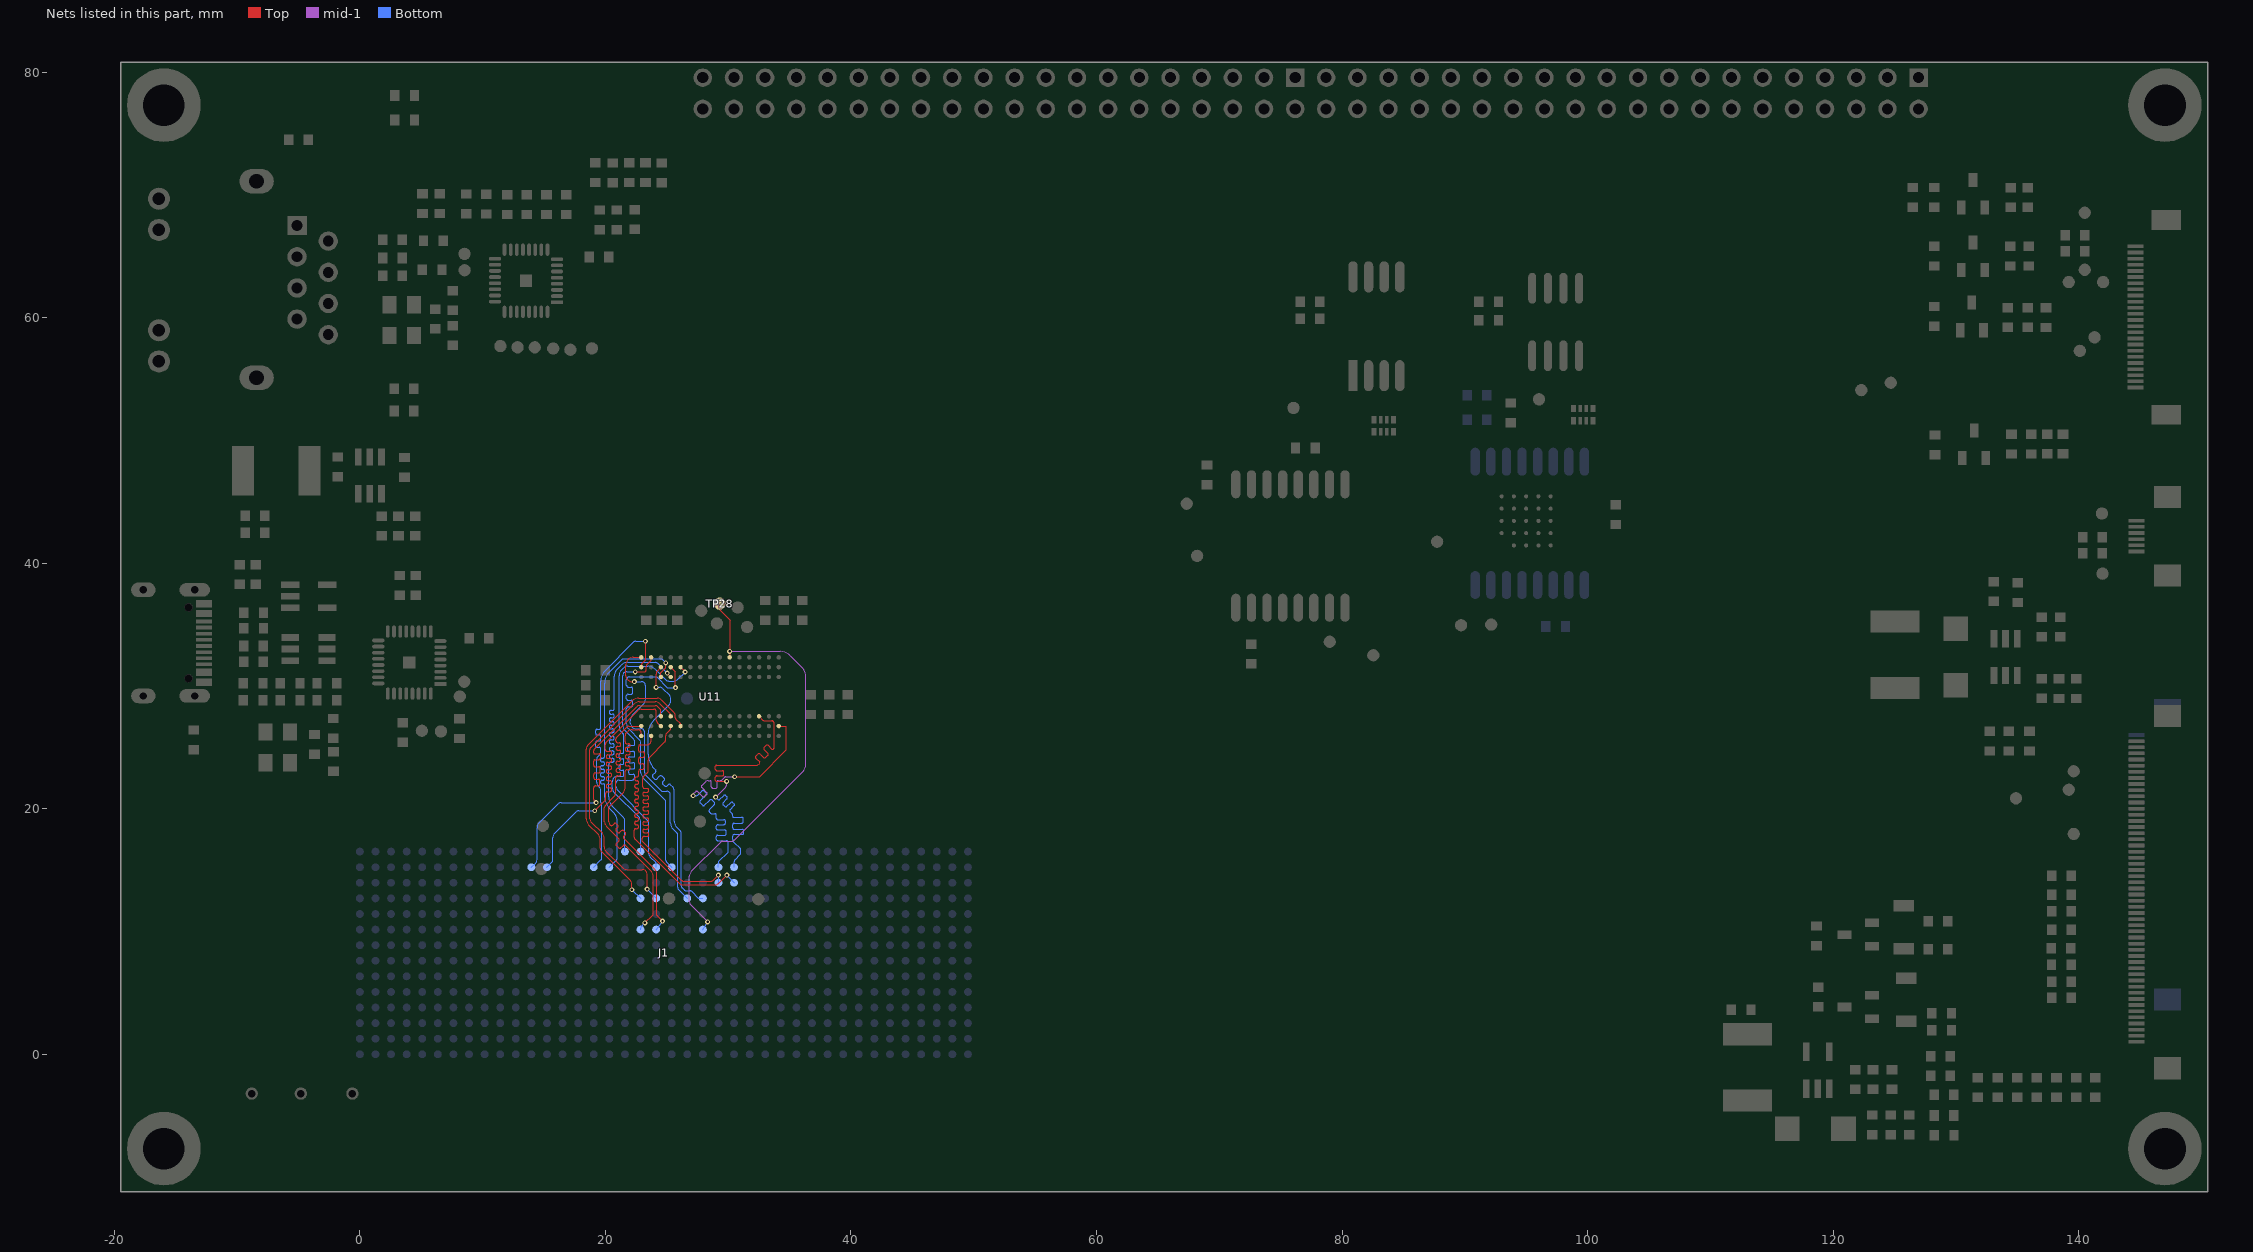
[diagram p0: the nets of this part, all layers, seen from the top]
# Altium PCB MISC105414.PcbDoc (part 10 of 11)
Units mm, origin at the board's own origin, x right, y up, seen from the top; angles counter-clockwise.
Board outline 170 x 92 mm, 6 copper layers (Top, GND, mid-1, mid-2, mid-3, Bottom), stack 1.231 mm thick; 238 components, 304 nets, 1456 pads, 1258 vias.
Unrouted connection lines stored in the file: 57.

## Via types
v1: diameter 0.4, hole 0.2, Top to Bottom, tented top, 618 vias
v2: diameter 0.5, hole 0.3, Top to Bottom, tented top, 522 vias
v3: diameter 0.5, hole 0.3, Top to Bottom, 41 vias
v4: diameter 1, hole 0.5, Top to Bottom, tented top, 36 vias
v5: diameter 0.7, hole 0.4, Top to Bottom, tented top, 34 vias
v6: diameter 1.3, hole 1.3, Top to Bottom, tented top, 3 vias
v7: diameter 4, hole 4, Top to Bottom, tented top, 2 vias
v8: diameter 3.3, hole 3.3, Top to Bottom, tented top, 2 vias

## Nets (pads, with @x,y where several pads share a name; then routed paths per layer and width w, separated by ;. In a path a pad name is that pad's centre, name@x,y a point inside that pad or via, vN(x,y) a via of type N, cw(c..) or ccw(c..) an arc to the next point about the centre after c; other vN are vias at no path point) (continued)
SDR_D14: J1.L16 U11.N3 | length 28.2
  Top w0.1: v1(29.874,22.224) 29.069,22.224 cw(c29.069,22.331) 28.962,22.331 28.962,22.558 cw(c29.098,22.558) 29.098,22.694 29.55,22.694 ccw(c29.55,22.788) 29.645,22.788 29.645,22.972 ccw(c29.516,22.972) 29.516,23.1 29.082,23.1 cw(c29.082,23.22) 28.962,23.22 28.962,23.454 cw(c29.054,23.454) 29.054,23.546 32.278,23.546 ccw(c32.278,23.875) 32.511,23.642 ; 32.511,23.642 32.556,23.688 ccw(c32.49,23.754) 32.584,23.754 ccw(c32.49,23.754) 32.556,23.82 32.25,24.126 cw(c32.333,24.21) 32.215,24.21 cw(c32.333,24.21) 32.25,24.293 32.417,24.46 cw(c32.504,24.372) 32.592,24.46 32.853,24.199 ccw(c32.96,24.306) 33.068,24.199 33.234,24.366 ccw(c33.163,24.437) 33.264,24.437 ccw(c33.163,24.437) 33.234,24.509 32.923,24.82 cw(c33.01,24.906) 32.887,24.906 cw(c33.01,24.906) 32.923,24.993 33.084,25.153 cw(c33.166,25.072) 33.247,25.153 33.527,24.874 ccw(c33.615,24.962) 33.739,24.962 33.739,26.975 ccw(c33.556,26.975) 33.556,27.158 32.982,27.158 cw(c32.982,27.369) 32.833,27.22 U11.N3@32.52,27.533
  mid-1 w0.1: v1(28.972,20.942) 29.79,21.76 ccw(c29.587,21.963) 29.874,21.963 v1(29.874,22.224)
  Bottom w0.1: v1(28.972,20.942) 29.157,20.757 ccw(c29.234,20.834) 29.311,20.757 29.622,21.067 cw(c29.714,20.976) 29.805,21.068 29.901,20.972 cw(c29.814,20.886) 29.937,20.886 cw(c29.814,20.886) 29.901,20.799 29.583,20.481 ccw(c29.658,20.406) 29.552,20.406 ccw(c29.658,20.406) 29.583,20.331 29.728,20.186 ccw(c29.814,20.272) 29.899,20.186 30.218,20.505 cw(c30.303,20.42) 30.387,20.505 30.501,20.391 cw(c30.448,20.338) 30.523,20.338 cw(c30.448,20.338) 30.501,20.285 30.151,19.935 ccw(c30.237,19.849) 30.116,19.849 ccw(c30.237,19.849) 30.151,19.763 30.149,19.761 30.311,19.598 cw(c30.195,19.482) 30.36,19.482 30.36,19.382 ccw(c30.442,19.382) 30.442,19.3 31.109,19.3 cw(c31.109,19.175) 31.234,19.175 31.234,18.967 cw(c31.098,18.967) 31.098,18.831 30.506,18.831 ccw(c30.506,18.685) 30.36,18.685 30.36,18.459 ccw(c30.501,18.459) 30.501,18.318 31.168,18.318 cw(c31.168,18.221) 31.265,18.221 31.265,18.017 cw(c31.155,18.017) 31.155,17.907 30.504,17.907 ccw(c30.504,17.763) 30.36,17.763 30.36,17.522 ccw(c30.722,17.522) 30.466,17.266 30.966,16.765 cw(c30.792,16.592) 31.038,16.592 31.038,16.42 cw(c30.832,16.42) 30.978,16.275 30.559,15.857 ccw(c30.75,15.666) 30.48,15.666 J1.L16@30.48,15.24
SDR_D15: J1.L17 U11.R2 | length 27.9
  Top w0.1: v1(30.517,22.609) 30.517,22.608 32.559,22.608 34.749,24.798 34.749,26.733 U11.R2@34.12,26.733
  mid-1 w0.1: v1(27.139,21.056) 27.139,21.097 cw(c27.357,21.097) 27.203,21.251 27.34,21.389 cw(c27.422,21.307) 27.503,21.389 27.886,21.006 ccw(c27.993,21.113) 28.1,21.006 28.273,21.179 ccw(c28.208,21.244) 28.3,21.244 ccw(c28.208,21.244) 28.273,21.309 27.843,21.74 cw(c27.918,21.815) 27.811,21.815 cw(c27.918,21.815) 27.842,21.891 28.156,22.205 cw(c28.371,21.989) 28.371,22.294 28.52,22.294 cw(c28.52,22.182) 28.632,22.182 28.632,21.776 ccw(c28.724,21.776) 28.724,21.684 29.025,21.684 ccw(c29.025,21.755) 29.096,21.755 29.096,22.206 cw(c29.184,22.206) 29.184,22.294 29.336,22.294 ccw(c29.336,22.522) 29.497,22.361 29.704,22.567 cw(c29.805,22.466) 29.805,22.609 v1(30.517,22.609)
  Bottom w0.1: v1(27.139,21.056) 27.375,21.056 ccw(c27.375,21.237) 27.503,21.109 27.839,21.445 cw(c27.949,21.335) 28.059,21.445 28.21,21.294 cw(c28.129,21.213) 28.243,21.213 cw(c28.129,21.213) 28.21,21.133 27.716,20.639 ccw(c27.796,20.559) 27.683,20.559 ccw(c27.796,20.559) 27.716,20.479 27.91,20.285 ccw(c27.99,20.364) 28.069,20.285 28.48,20.696 cw(c28.592,20.583) 28.705,20.696 28.868,20.533 cw(c28.769,20.434) 28.909,20.434 cw(c28.769,20.434) 28.868,20.335 28.479,19.946 ccw(c28.594,19.831) 28.431,19.831 ccw(c28.594,19.831) 28.479,19.716 28.531,19.664 ccw(c28.697,19.829) 28.697,19.595 28.908,19.595 cw(c28.908,19.466) 29.038,19.466 29.038,19.213 ccw(c29.138,19.213) 29.138,19.113 29.644,19.113 cw(c29.644,18.976) 29.781,18.976 29.781,18.853 cw(c29.643,18.853) 29.643,18.714 29.185,18.714 ccw(c29.185,18.567) 29.038,18.567 29.038,18.385 ccw(c29.148,18.385) 29.148,18.275 29.707,18.275 cw(c29.707,18.14) 29.842,18.14 29.842,17.963 cw(c29.734,17.963) 29.734,17.855 29.156,17.855 ccw(c29.156,17.736) 29.038,17.736 29.038,17.505 ccw(c29.13,17.505) 29.13,17.413 29.856,17.413 cw(c29.856,17.276) 29.993,17.276 29.993,16.457 29.246,15.71 J1.L17@29.21,15.24
SDR_D16: J1.M22 U11.E8 | length 24.4
  Top w0.1: U11.E8@26.12,31.533 26.488,31.165 v1(26.488,31.139)
  Bottom w0.1: J1.M22@22.86,16.51 22.86,19.028 ccw(c22.461,19.028) 22.743,19.31 20.695,21.358 cw(c21.029,21.693) 20.557,21.693 20.557,22.196 cw(c20.995,22.196) 20.995,22.634 21.393,22.634 ccw(c21.393,22.751) 21.509,22.751 21.509,23.054 ccw(c21.407,23.054) 21.407,23.157 21.238,23.157 cw(c21.238,23.278) 21.117,23.278 21.117,23.494 cw(c21.24,23.494) 21.24,23.617 21.399,23.617 ccw(c21.399,23.727) 21.509,23.727 21.509,23.962 ccw(c21.4,23.962) 21.4,24.072 21.214,24.072 cw(c21.214,24.164) 21.121,24.164 21.121,24.435 cw(c21.215,24.435) 21.215,24.529 21.401,24.529 ccw(c21.401,24.637) 21.509,24.637 21.509,25.913 ccw(c21.206,25.913) 21.42,26.128 21.315,26.233 cw(c21.811,26.728) 21.11,26.728 21.11,30.85 cw(c21.703,30.85) 21.284,31.269 21.5,31.486 cw(c21.814,31.172) 21.814,31.616 23.462,31.616 cw(c23.462,30.798) 24.04,31.376 24.902,30.514 ccw(c25.164,30.775) 25.164,30.405 25.569,30.405 ccw(c25.569,30.851) 25.884,30.536 v1(26.488,31.139)
SDR_D17: J1.M23 U11.D7 | length 24.8
  Top w0.1: v1(25.038,31.052) 25.038,31.014 U11.D7@25.32,30.733
  Bottom w0.1: J1.M23@21.59,16.51 21.59,18.994 ccw(c21.155,18.994) 21.463,19.302 20.574,20.19 cw(c21.346,20.962) 20.255,20.962 20.255,23.592 cw(c20.469,23.592) 20.469,23.806 20.57,23.806 ccw(c20.57,23.956) 20.72,23.956 ccw(c20.57,23.956) 20.57,24.106 20.457,24.106 cw(c20.457,24.256) 20.307,24.256 cw(c20.457,24.256) 20.457,24.406 20.57,24.406 ccw(c20.57,24.556) 20.72,24.556 ccw(c20.57,24.556) 20.57,24.706 20.457,24.706 cw(c20.457,24.856) 20.307,24.856 cw(c20.457,24.856) 20.457,25.006 20.57,25.006 ccw(c20.57,25.156) 20.72,25.156 ccw(c20.57,25.156) 20.57,25.306 20.457,25.306 cw(c20.457,25.456) 20.307,25.456 cw(c20.457,25.456) 20.457,25.606 20.57,25.606 ccw(c20.57,25.756) 20.72,25.756 ccw(c20.57,25.756) 20.57,25.906 20.457,25.906 cw(c20.457,26.056) 20.307,26.056 cw(c20.457,26.056) 20.457,26.206 20.57,26.206 ccw(c20.57,26.356) 20.72,26.356 ccw(c20.57,26.356) 20.57,26.506 20.457,26.506 cw(c20.457,26.656) 20.307,26.656 cw(c20.457,26.656) 20.457,26.806 20.57,26.806 ccw(c20.57,26.956) 20.72,26.956 ccw(c20.57,26.956) 20.57,27.106 20.457,27.106 cw(c20.457,27.256) 20.307,27.256 cw(c20.457,27.256) 20.457,27.406 20.57,27.406 ccw(c20.57,27.556) 20.72,27.556 ccw(c20.57,27.556) 20.57,27.706 20.457,27.706 cw(c20.457,27.856) 20.307,27.856 cw(c20.457,27.856) 20.457,28.006 20.57,28.006 ccw(c20.57,28.156) 20.72,28.156 20.72,30.784 cw(c21.56,30.784) 20.966,31.378 21.289,31.701 cw(c21.809,31.182) 21.809,31.916 24.063,31.916 cw(c24.063,31.648) 24.253,31.838 v1(25.038,31.052)
SDR_D18: J1.L20 U11.D8 | length 24.6
  Top w0.1: U11.D8@25.32,31.533 25.7,31.153 25.7,29.867 v1(25.71,29.867)
  Bottom w0.1: J1.L20@25.4,15.24 24.992,15.648 cw(c25.141,15.798) 24.93,15.798 24.93,20.532 ccw(c24.653,20.532) 24.849,20.727 23.05,22.526 cw(c23.451,22.927) 22.884,22.927 22.884,25.347 ccw(c22.481,25.347) 22.766,25.632 21.894,26.505 cw(c22.322,26.932) 21.717,26.932 21.717,28.159 cw(c21.872,28.159) 21.872,28.314 22.121,28.314 ccw(c22.121,28.401) 22.209,28.401 22.209,28.723 ccw(c22.093,28.723) 22.093,28.839 21.825,28.839 cw(c21.825,28.947) 21.717,28.947 21.717,29.204 cw(c21.853,29.204) 21.853,29.341 22.119,29.341 ccw(c22.119,29.441) 22.219,29.441 22.219,29.783 ccw(c22.095,29.783) 22.095,29.908 21.883,29.908 cw(c21.883,30.073) 21.717,30.073 21.717,30.503 cw(c21.96,30.503) 21.96,30.746 24.164,30.746 25.043,29.867 v1(25.71,29.867)
SDR_D19: J1.L21 U11.B9 | length 24.6
  Top w0.1: v1(22.428,31.151) 23.183,31.151 ccw(c23.183,31.287) 23.32,31.287 23.32,31.599 cw(c23.514,31.599) 23.377,31.737 23.689,32.049 ; 23.689,32.049 ccw(c23.614,32.124) 23.72,32.124 U11.B9@23.72,32.333
  Bottom w0.1: v1(22.428,31.151) 21.723,31.151 ccw(c21.723,30.838) 21.41,30.838 21.41,26.776 ccw(c21.926,26.776) 21.561,26.412 22.253,25.72 cw(c21.914,25.381) 22.394,25.381 22.394,25.255 cw(c22.306,25.255) 22.306,25.167 21.947,25.167 ccw(c21.947,25.03) 21.81,25.03 21.81,24.77 ccw(c21.912,24.77) 21.912,24.668 22.237,24.668 cw(c22.237,24.511) 22.394,24.511 22.394,24.303 cw(c22.308,24.303) 22.308,24.217 21.94,24.217 ccw(c21.94,24.124) 21.846,24.124 21.846,23.862 ccw(c21.942,23.862) 21.942,23.766 22.243,23.766 cw(c22.243,23.615) 22.394,23.615 22.394,23.378 cw(c22.257,23.378) 22.257,23.241 22.032,23.241 ccw(c22.032,23.091) 21.882,23.091 21.882,22.916 ccw(c21.999,22.916) 21.999,22.8 22.267,22.8 cw(c22.267,22.673) 22.394,22.673 22.394,22.579 cw(c22.148,22.579) 22.148,22.333 21.125,22.333 ccw(c21.125,22.066) 20.857,22.066 20.857,21.835 ccw(c21.303,21.835) 20.988,21.52 23.468,19.04 cw(c23.312,18.884) 23.532,18.884 23.532,16.348 ccw(c23.868,16.348) 23.63,16.11 24.094,15.647 cw(c24.006,15.559) 24.13,15.559 J1.L21@24.13,15.24
SDR_D20: J1.J18 U11.C8 | length 24.1
  Top w0.1: v1(24.128,29.888) 24.129,29.849 24.129,30.976 cw(c24.529,30.976) 24.246,31.259 U11.C8@24.52,31.533
  Bottom w0.1: v1(24.128,29.888) 24.443,29.888 cw(c24.443,29.55) 24.681,29.789 25.199,29.271 cw(c24.912,28.985) 25.317,28.985 25.317,28.735 cw(c24.971,28.735) 25.216,28.49 23.926,27.2 ccw(c24.972,26.154) 23.492,26.154 23.492,24.448 ccw(c25.15,24.448) 23.978,23.276 24.079,23.174 cw(c23.977,23.072) 24.122,23.072 cw(c23.977,23.072) 24.079,22.969 23.867,22.756 ccw(c23.966,22.657) 23.825,22.657 ccw(c23.966,22.657) 23.867,22.558 24.003,22.422 ccw(c24.094,22.514) 24.186,22.422 24.397,22.633 cw(c24.509,22.521) 24.621,22.633 ; 24.621,22.633 24.788,22.465 cw(c24.709,22.386) 24.821,22.386 cw(c24.709,22.386) 24.788,22.306 24.68,22.198 ccw(c24.782,22.096) 24.638,22.096 ccw(c24.782,22.096) 24.68,21.994 24.815,21.859 ccw(c24.921,21.966) 25.028,21.859 25.121,21.953 cw(c25.211,21.863) 25.301,21.953 25.478,21.776 ; 25.478,21.776 cw(c25.181,21.478) 25.601,21.478 25.601,18.985 ccw(c26.302,18.985) 25.807,18.489 26.099,18.196 cw(c25.907,18.004) 26.179,18.004 26.179,13.712 ccw(c26.406,13.712) 26.246,13.551 26.403,13.394 ccw(c26.582,13.572) 26.582,13.32 26.879,13.32 cw(c26.879,13.128) 27.015,13.263 27.528,12.75 ccw(c27.648,12.87) 27.648,12.7 J1.J18@27.94,12.7
SDR_D21: J1.J19 U11.A9 | length 24.8
  Top w0.1: v1(22.364,30.357) 22.146,30.357 cw(c22.146,30.843) 21.661,30.843 21.661,31.724 cw(c22.27,31.724) 22.27,32.333 U11.A9@22.92,32.333
  Bottom w0.1: v1(22.364,30.357) 22.931,30.357 cw(c22.931,30.021) 23.267,30.021 23.267,28.939 cw(c22.686,28.939) 23.097,28.529 22.237,27.669 ccw(c22.73,27.176) 22.033,27.176 22.033,26.985 ccw(c22.499,26.985) 22.499,26.518 22.893,26.518 cw(c22.893,26.222) 23.189,26.222 23.189,22.924 ccw(c23.461,22.924) 23.269,22.731 24.57,21.431 24.993,21.431 cw(c24.993,21.13) 25.294,21.13 25.294,18.841 ccw(c25.934,18.841) 25.481,18.389 25.827,18.043 cw(c25.703,17.918) 25.879,17.918 25.879,13.61 ccw(c26.164,13.61) 25.962,13.408 J1.J19@26.67,12.7
SDR_D22: J1.L24 U11.C7 | length 24.9
  Top w0.1: U11.C7@24.52,30.733 24.52,31.069 24.926,31.475 24.926,31.872 v1(24.916,31.881)
  Bottom w0.1: J1.L24@20.32,15.24 20.87,15.79 ccw(c20.613,16.047) 20.977,16.047 20.977,19.004 ccw(c20.109,19.004) 20.723,19.617 20.345,19.995 cw(c21.289,20.939) 19.954,20.939 19.954,21.925 ccw(c19.858,21.925) 19.858,22.02 19.733,22.02 cw(c19.733,22.17) 19.583,22.17 cw(c19.733,22.17) 19.733,22.32 19.788,22.32 ccw(c19.788,22.47) 19.938,22.47 ccw(c19.788,22.47) 19.788,22.62 19.733,22.62 cw(c19.733,22.77) 19.583,22.77 cw(c19.733,22.77) 19.733,22.92 19.788,22.92 ccw(c19.788,23.07) 19.938,23.07 ccw(c19.788,23.07) 19.788,23.22 19.733,23.22 cw(c19.733,23.37) 19.583,23.37 cw(c19.733,23.37) 19.733,23.52 19.788,23.52 ccw(c19.788,23.67) 19.938,23.67 ccw(c19.788,23.67) 19.788,23.82 19.733,23.82 cw(c19.733,23.97) 19.583,23.97 cw(c19.733,23.97) 19.733,24.12 19.788,24.12 ccw(c19.788,24.27) 19.938,24.27 19.938,30.241 cw(c21.139,30.241) 20.29,31.091 21.419,32.219 24.578,32.219 v1(24.916,31.881)
SDR_D23: J1.L25 U11.A8 | length 24.5
  Top w0.1: U11.A8@22.92,31.533 22.92,31.709 cw(c23.059,31.709) 22.961,31.807 23.234,32.08 ccw(c23.094,32.221) 23.292,32.221 23.292,33.484 23.3,33.491 23.279,33.512 23.269,33.565 v1(23.253,33.648)
  Bottom w0.1: J1.L25@19.05,15.24 19.64,15.83 ccw(c19.449,16.021) 19.719,16.021 19.719,20.309 ccw(c19.57,20.309) 19.675,20.414 19.667,20.421 cw(c19.772,20.526) 19.624,20.526 19.624,21.49 ccw(c19.255,21.49) 19.516,21.751 19.397,21.87 cw(c19.688,22.161) 19.276,22.161 19.276,24.037 cw(c19.574,24.037) 19.363,24.247 19.525,24.409 ccw(c19.311,24.622) 19.613,24.622 19.613,24.9 ccw(c19.511,24.9) 19.511,25.002 19.274,25.002 cw(c19.274,25.081) 19.195,25.081 19.195,25.386 cw(c19.328,25.386) 19.328,25.52 19.509,25.52 ccw(c19.509,25.648) 19.638,25.648 19.638,25.91 ccw(c19.537,25.91) 19.537,26.011 19.319,26.011 cw(c19.319,26.134) 19.196,26.134 19.196,26.358 cw(c19.323,26.358) 19.323,26.485 19.516,26.485 ccw(c19.516,26.583) 19.613,26.583 19.613,30.391 cw(c20.78,30.391) 19.955,31.216 22.328,33.589 cw(c22.469,33.447) 22.469,33.648 v1(23.253,33.648)
SDR_D24: J1.G22 U11.A2 | length 24.1
  Top w0.1: U11.A2@22.92,26.733 21.916,26.733 ccw(c21.916,26.523) 21.768,26.671 20.905,25.809 ccw(c21.043,25.671) 20.848,25.671 20.848,25.539 20.855,25.531 ccw(c21.005,25.531) 21.005,25.381 21.115,25.381 cw(c21.115,25.231) 21.265,25.231 cw(c21.115,25.231) 21.115,25.081 21.005,25.081 ccw(c21.005,24.931) 20.855,24.931 ccw(c21.005,24.931) 21.005,24.781 21.115,24.781 cw(c21.115,24.631) 21.265,24.631 cw(c21.115,24.631) 21.115,24.481 21.005,24.481 ccw(c21.005,24.331) 20.855,24.331 ccw(c21.005,24.331) 21.005,24.181 21.115,24.181 cw(c21.115,24.031) 21.265,24.031 cw(c21.115,24.031) 21.115,23.881 21.005,23.881 ccw(c21.005,23.731) 20.855,23.731 ccw(c21.005,23.731) 21.005,23.581 21.115,23.581 cw(c21.115,23.431) 21.265,23.431 cw(c21.115,23.431) 21.115,23.281 21.005,23.281 ccw(c21.005,23.131) 20.855,23.131 ccw(c21.005,23.131) 21.005,22.981 21.115,22.981 cw(c21.115,22.831) 21.265,22.831 cw(c21.115,22.831) 21.115,22.681 20.999,22.681 ccw(c20.999,22.531) 20.849,22.531 20.849,21.365 cw(c20.274,21.365) 20.681,20.959 20.012,20.291 ccw(c20.232,20.071) 19.921,20.071 19.921,18.951 ccw(c20.436,18.951) 20.072,18.587 21.089,17.57 cw(c20.982,17.464) 21.133,17.464 cw(c20.982,17.464) 21.089,17.357 20.871,17.139 ccw(c20.935,17.074) 20.844,17.074 ccw(c20.935,17.074) 20.871,17.01 21.069,16.812 ccw(c21.16,16.903) 21.251,16.812 21.436,16.997 cw(c21.549,16.884) 21.662,16.997 23.701,14.958 cw(c23.22,14.478) 23.9,14.478 23.9,11.465 cw(c23.688,11.465) 23.838,11.315 v1(23.221,10.698)
  Bottom w0.1: J1.G22@22.86,10.16 22.86,10.268 cw(c23.026,10.268) 22.909,10.385 v1(23.221,10.698)
SDR_D25: J1.L29 U11.C3 | length 23.8
  Top w0.1: v1(19.242,20.501) 19.072,20.671 cw(c19.175,20.774) 19.029,20.774 19.029,21.692 cw(c19.193,21.692) 19.193,21.856 19.413,21.856 ccw(c19.413,21.989) 19.545,21.989 19.545,22.293 ccw(c19.431,22.293) 19.431,22.408 19.169,22.408 cw(c19.169,22.547) 19.029,22.547 19.029,22.779 cw(c19.172,22.779) 19.172,22.922 19.475,22.922 ccw(c19.475,23.02) 19.572,23.02 19.572,23.332 ccw(c19.471,23.332) 19.471,23.433 19.133,23.433 cw(c19.133,23.537) 19.029,23.537 19.029,23.877 cw(c19.148,23.877) 19.148,23.995 19.44,23.995 ccw(c19.44,24.155) 19.6,24.155 19.6,24.387 ccw(c19.495,24.387) 19.495,24.493 19.096,24.493 cw(c19.096,24.559) 19.029,24.559 19.029,24.712 cw(c19.2,24.712) 19.079,24.833 22.564,28.318 cw(c22.782,28.1) 22.782,28.408 24.079,28.408 cw(c24.079,28.192) 24.232,28.345 24.436,28.141 cw(c24.232,27.937) 24.52,27.937 U11.C3@24.52,27.533
  Bottom w0.1: J1.L29@13.97,15.24 14.308,15.578 ccw(c13.986,15.899) 14.441,15.899 14.441,18.47 cw(c14.986,18.47) 14.601,18.856 16.146,20.401 cw(c16.388,20.16) 16.388,20.501 v1(19.242,20.501)
SDR_D26: J1.G21 U11.A1 | length 23.8
  Top w0.1: 20.871,18.213 21.007,18.077 ccw(c21.091,18.162) 21.175,18.077 21.301,18.203 cw(c21.397,18.106) 21.493,18.203 21.634,18.062 cw(c21.546,17.973) 21.671,17.973 cw(c21.546,17.973) 21.634,17.885 21.503,17.754 ccw(c21.59,17.668) 21.467,17.668 ccw(c21.59,17.668) 21.503,17.581 24.01,15.074 cw(c23.551,14.615) 24.2,14.615 24.2,11.345 ccw(c24.309,11.345) 24.232,11.268 v1(24.65,10.85) ; 20.87,18.213 cw(c20.946,18.289) 20.839,18.289 cw(c20.946,18.289) 20.871,18.364 21.005,18.498 ccw(c20.925,18.578) 21.038,18.578 ccw(c20.925,18.578) 21.005,18.658 20.87,18.793 ccw(c20.791,18.714) 20.712,18.793 20.59,18.671 cw(c20.501,18.759) 20.413,18.67 20.367,18.717 cw(c20.577,18.928) 20.279,18.928 20.279,20.035 cw(c20.518,20.035) 20.349,20.203 21.406,21.26 ccw(c20.898,21.769) 21.617,21.769 21.617,23.042 cw(c21.767,23.042) 21.767,23.192 21.869,23.192 ccw(c21.869,23.342) 22.019,23.342 ccw(c21.869,23.342) 21.869,23.492 21.746,23.492 cw(c21.746,23.642) 21.596,23.642 cw(c21.746,23.642) 21.746,23.792 21.869,23.792 ccw(c21.869,23.942) 22.019,23.942 ccw(c21.869,23.942) 21.869,24.092 21.746,24.092 cw(c21.746,24.242) 21.596,24.242 cw(c21.746,24.242) 21.746,24.392 21.869,24.392 ccw(c21.869,24.542) 22.019,24.542 ccw(c21.869,24.542) 21.869,24.692 21.746,24.692 cw(c21.746,24.842) 21.596,24.842 cw(c21.746,24.842) 21.746,24.992 21.869,24.992 ccw(c21.869,25.142) 22.019,25.142 ccw(c21.869,25.142) 21.869,25.292 21.746,25.292 cw(c21.746,25.442) 21.596,25.442 21.596,25.964 cw(c21.861,25.964) 21.673,26.152 21.803,26.282 cw(c22.191,25.858) 22.191,26.433 22.674,26.433 cw(c22.674,26.186) 22.92,26.186 U11.A1@22.92,25.933
  Bottom w0.1: J1.G21@24.13,10.16 v1(24.65,10.85)
SDR_D27: J1.L28 U11.C2 | length 23.7
  Top w0.1: v1(19.133,19.836) 19.975,20.678 ccw(c19.869,20.785) 20.019,20.785 20.019,21.247 cw(c20.169,21.247) 20.169,21.397 20.363,21.397 ccw(c20.363,21.547) 20.513,21.547 ccw(c20.363,21.547) 20.363,21.697 20.198,21.697 cw(c20.198,21.847) 20.048,21.847 cw(c20.198,21.847) 20.198,21.997 20.363,21.997 ccw(c20.363,22.147) 20.513,22.147 ccw(c20.363,22.147) 20.363,22.297 20.198,22.297 cw(c20.198,22.447) 20.048,22.447 cw(c20.198,22.447) 20.198,22.597 20.363,22.597 ccw(c20.363,22.747) 20.513,22.747 ccw(c20.363,22.747) 20.363,22.897 20.198,22.897 cw(c20.198,23.047) 20.048,23.047 cw(c20.198,23.047) 20.198,23.197 20.363,23.197 ccw(c20.363,23.347) 20.513,23.347 ccw(c20.363,23.347) 20.363,23.497 20.198,23.497 cw(c20.198,23.647) 20.048,23.647 cw(c20.198,23.647) 20.198,23.797 20.363,23.797 ccw(c20.363,23.947) 20.513,23.947 ccw(c20.363,23.947) 20.363,24.097 20.198,24.097 cw(c20.198,24.247) 20.048,24.247 cw(c20.198,24.247) 20.198,24.397 20.363,24.397 ccw(c20.363,24.547) 20.513,24.547 ccw(c20.363,24.547) 20.363,24.697 20.122,24.697 cw(c20.122,24.847) 19.972,24.847 19.972,25.203 cw(c20.206,25.203) 20.04,25.368 22.694,28.022 cw(c22.899,27.816) 22.899,28.107 23.95,28.107 cw(c23.95,27.907) 24.15,27.907 24.15,27.221 ccw(c24.435,27.221) 24.233,27.019 U11.C2@24.52,26.733
  Bottom w0.1: J1.L28@15.24,15.24 15.714,15.714 15.714,17.654 cw(c16.169,17.654) 15.847,17.976 17.617,19.746 cw(c17.833,19.53) 17.833,19.836 v1(19.133,19.836)
SDR_D28: J1.K16 U11.B1 | length 24
  Top w0.1: 22.518,19.288 22.554,19.288 cw(c22.554,19.138) 22.704,19.138 cw(c22.554,19.138) 22.554,18.988 22.518,18.988 ccw(c22.518,18.838) 22.368,18.838 ccw(c22.518,18.838) 22.518,18.688 22.554,18.688 cw(c22.554,18.538) 22.704,18.538 cw(c22.554,18.538) 22.554,18.388 22.482,18.388 ccw(c22.482,18.238) 22.332,18.238 22.332,17.671 ccw(c22.495,17.671) 22.379,17.556 25.962,13.973 ccw(c26.389,14.399) 26.389,13.796 28.934,13.796 ccw(c28.934,14.188) 29.211,13.911 v1(29.9,14.6) ; 22.518,19.288 cw(c22.518,19.438) 22.368,19.438 cw(c22.518,19.438) 22.518,19.588 22.554,19.588 ccw(c22.554,19.738) 22.704,19.738 ccw(c22.554,19.738) 22.554,19.888 22.518,19.888 cw(c22.518,20.038) 22.368,20.038 cw(c22.518,20.038) 22.518,20.188 22.554,20.188 ccw(c22.554,20.338) 22.704,20.338 ccw(c22.554,20.338) 22.554,20.488 22.518,20.488 cw(c22.518,20.638) 22.368,20.638 cw(c22.518,20.638) 22.518,20.788 22.554,20.788 ccw(c22.554,20.938) 22.704,20.938 ccw(c22.554,20.938) 22.554,21.088 22.518,21.088 cw(c22.518,21.238) 22.368,21.238 cw(c22.518,21.238) 22.518,21.388 22.554,21.388 ccw(c22.554,21.538) 22.704,21.538 ccw(c22.554,21.538) 22.554,21.688 22.518,21.688 cw(c22.518,21.838) 22.368,21.838 cw(c22.518,21.838) 22.518,21.988 22.554,21.988 ccw(c22.554,22.138) 22.704,22.138 ccw(c22.554,22.138) 22.554,22.288 22.518,22.288 cw(c22.518,22.438) 22.368,22.438 cw(c22.518,22.438) 22.518,22.588 22.554,22.588 ccw(c22.554,22.738) 22.704,22.738 22.704,23.07 cw(c22.841,23.07) 22.841,23.207 22.992,23.207 ccw(c22.992,23.369) 23.154,23.369 23.154,23.533 ccw(c23.013,23.533) 23.013,23.675 22.805,23.675 cw(c22.805,23.775) 22.704,23.775 22.704,24.087 cw(c22.81,24.087) 22.81,24.193 23.067,24.193 ccw(c23.067,24.311) 23.185,24.311 23.185,24.521 ccw(c23.069,24.521) 23.069,24.636 22.784,24.636 cw(c22.784,24.716) 22.704,24.716 22.704,25.067 cw(c22.85,25.067) 22.85,25.213 23.389,25.213 ccw(c23.389,25.544) 23.72,25.544 U11.B1@23.72,25.933
  Bottom w0.1: v1(29.9,14.6) J1.K16@30.48,13.97
SDR_D29: J1.K17 U11.D2 | length 24.1
  Top w0.1: 23.183,21.65 23.399,21.65 cw(c23.399,21.5) 23.549,21.5 cw(c23.399,21.5) 23.399,21.35 23.183,21.35 ccw(c23.183,21.2) 23.033,21.2 ccw(c23.183,21.2) 23.183,21.05 23.399,21.05 cw(c23.399,20.9) 23.549,20.9 cw(c23.399,20.9) 23.399,20.75 23.183,20.75 ccw(c23.183,20.6) 23.033,20.6 ccw(c23.183,20.6) 23.183,20.45 23.399,20.45 cw(c23.399,20.3) 23.549,20.3 cw(c23.399,20.3) 23.399,20.15 23.183,20.15 ccw(c23.183,20) 23.033,20 ccw(c23.183,20) 23.183,19.85 23.399,19.85 cw(c23.399,19.7) 23.549,19.7 cw(c23.399,19.7) 23.399,19.55 23.183,19.55 ccw(c23.183,19.4) 23.033,19.4 ccw(c23.183,19.4) 23.183,19.25 23.399,19.25 cw(c23.399,19.1) 23.549,19.1 cw(c23.399,19.1) 23.399,18.95 23.183,18.95 ccw(c23.183,18.8) 23.033,18.8 ccw(c23.183,18.8) 23.183,18.65 23.399,18.65 cw(c23.399,18.5) 23.549,18.5 cw(c23.399,18.5) 23.399,18.35 23.183,18.35 ccw(c23.183,18.2) 23.033,18.2 ccw(c23.183,18.2) 23.183,18.05 23.399,18.05 cw(c23.399,17.9) 23.549,17.9 cw(c23.399,17.9) 23.399,17.75 23.157,17.75 ccw(c23.157,17.6) 23.007,17.6 23.007,17.353 26.165,14.194 ccw(c26.401,14.43) 26.401,14.097 28.616,14.097 ccw(c28.616,14.307) 28.765,14.159 v1(29.197,14.59) ; 23.183,21.65 cw(c23.183,21.8) 23.033,21.8 23.033,22.439 cw(c23.265,22.439) 23.101,22.603 23.417,22.92 ccw(c23.24,23.097) 23.491,23.097 23.491,23.943 cw(c23.86,23.943) 23.599,24.204 24.84,25.445 ccw(c24.694,25.591) 24.9,25.591 24.9,25.953 cw(c25.158,25.953) 24.976,26.135 25.281,26.44 ; 25.281,26.44 ccw(c25.186,26.535) 25.32,26.535 U11.D2@25.32,26.733
  Bottom w0.1: v1(29.197,14.59) J1.K17@29.21,13.97
SDR_D30: J1.J21 U11.D3 | length 23.9
  Top w0.1: v1(23.4,13.45) 23.4,14.653 ccw(c23.005,14.653) 23.005,15.048 21.785,15.048 cw(c21.785,15.632) 21.371,15.219 20.047,16.543 cw(c20.401,16.897) 19.901,16.897 19.901,17.606 ccw(c19.306,17.606) 19.726,18.027 18.848,18.905 cw(c19.137,19.193) 18.729,19.193 18.729,24.798 cw(c18.997,24.798) 18.808,24.987 22.36,28.539 cw(c22.769,28.13) 22.769,28.709 24.077,28.709 cw(c24.077,28.19) 24.444,28.557 25.32,27.681 U11.D3@25.32,27.533
  Bottom w0.1: v1(23.4,13.45) J1.J21@24.13,12.7
SDR_D31: J1.J22 U11.E2 | length 24.6
  Top w0.1: v1(22.15,13.4) 22.15,13.818 ccw(c21.67,13.818) 22.009,14.157 19.688,16.478 cw(c19.979,16.769) 19.568,16.769 19.568,17.487 ccw(c18.906,17.487) 19.374,17.955 18.621,18.708 cw(c19.085,19.172) 18.428,19.172 18.428,24.848 cw(c18.874,24.848) 18.559,25.163 22.189,28.793 cw(c22.711,28.271) 22.711,29.009 24.205,29.009 cw(c24.205,28.497) 24.568,28.859 25.569,27.858 cw(c25.264,27.552) 25.696,27.552 25.696,27.394 ccw(c25.815,27.394) 25.731,27.31 26.093,26.948 cw(c26.026,26.882) 26.12,26.882 U11.E2@26.12,26.733
  Bottom w0.1: v1(22.15,13.4) J1.J22@22.86,12.7
SDR_DQM0: J1.G18 TP28.1 U11.K9 | length 37.7
  Top w0.1: TP28.1@29.312,36.708 29.312,36.215 30.178,35.349 30.178,32.873 v1(30.117,32.812) U11.K9@30.12,32.333
  mid-1 w0.1: v1(28.33,10.789) 26.975,12.145 cw(c27.31,12.48) 26.836,12.48 26.836,14.511 cw(c27.393,14.511) 26.999,14.905 29.379,17.285 cw(c29.539,17.125) 29.539,17.352 30.283,17.352 ccw(c30.283,17.63) 30.48,17.433 36.119,23.072 ccw(c35.614,23.577) 36.328,23.577 36.328,30.705 ccw(c35.096,30.705) 35.967,31.576 35.075,32.469 ccw(c34.246,31.64) 34.246,32.812 v1(30.117,32.812)
  Bottom w0.1: J1.G18@27.94,10.16 v1(28.33,10.789)